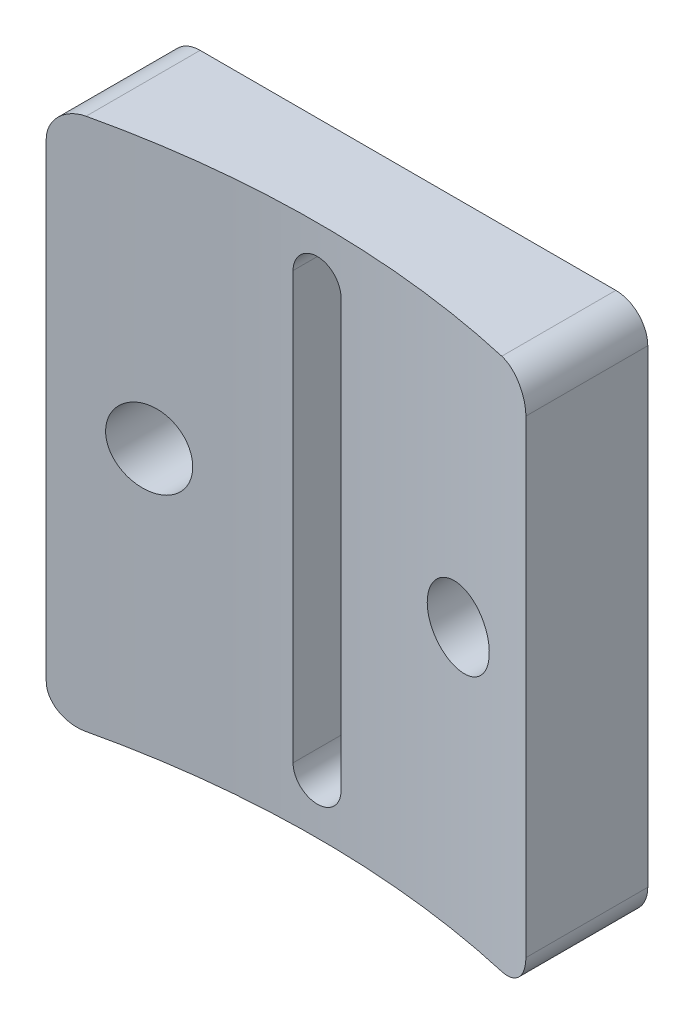
SolidWorks part; units mm, degrees
ref_plane "Front Plane" through (0, 0, 0) normal (0, 0, 1) x (1, 0, 0)
ref_plane "Top Plane" through (0, 0, 0) normal (0, 1, 0) x (1, 0, 0)
ref_plane "Right Plane" through (0, 0, 0) normal (1, 0, 0) x (0, 0, -1)
sketch "Sketch1" plane through (0, 0, 0) normal (0, 1, 0) x (1, 0, 0)
  line L0 (-22.5, 84.5577) -> (-22.5, 96)
  line L1 (-22.5, 96) -> (22.5, 96)
  line L2 (22.5, 96) -> (22.5, 84.5577)
  line L3 (0, 0) -> (0, 120.121) construction
  arc A0 (22.5, 84.5577) -> (-22.5, 84.5577) centre (0, 0) ccw
  dimension "D1" = 175
  dimension "D2" = 45
  dimension "D4" = 96
extrude "Boss-Extrude1" add sketch "Sketch1" along normal blind 50
hole_wizard "M8x1.0 Tapped Hole1" positions "Sketch3" profile "Sketch2" tap size "M8x1.0" standard "GB" end condition through all
sketch "Sketch3" plane through (0, 0, -96) normal (0, 0, -1) x (-1, 0, 0)
  line L0 (-22.5, 0) -> (22.5, 0) construction
  line L1 (22.5, 50) -> (-22.5, 50) construction
  line L2 (-22.5, 50) -> (-22.5, 0) construction
  line L3 (22.5, 50) -> (22.5, 0) construction
  point P0 (-14.5, 25)
  point P2 (14.5, 25)
  point P5 (0, 0)
  point P8 (0, 50)
  point P11 (-22.5, 25)
  point P14 (22.5, 25)
  dimension "D1" = 14.5
  dimension "D2" = 14.5
  dimension "D3" = 0
  dimension "D4" = 0
sketch "Sketch2" plane through (14.5, 25, -96) normal (1, 0, 0) x (0, 1, 0)
  line L0 (0, 0) -> (0, 11.4423)
  line L1 (0, 11.4423) -> (3.5, 11.4423)
  line L2 (3.5, 11.4423) -> (3.5, 0)
  line L5 (3.5, 0) -> (0, 0)
  line L11 (0, -6.35) -> (0, 107.95) construction
  dimension "通孔螺纹孔钻头直径" = 7
  dimension "通孔螺纹孔钻头深度" = 11.4423
cosmetic thread "Cosmetic thread 1" parameters "D1"=8.0513, "D2"=8
cosmetic thread "Cosmetic thread 2" parameters "D1"=8.0513, "D2"=8
sketch "Sketch4" plane through (0, 0, -96) normal (0, 0, -1) x (-1, 0, 0)
  line L0 (0, 0) -> (0, 35.1081) construction
  line L2 (-22.5, 25) -> (24.5658, 25) construction
  line L3 (-22.5, 50) -> (-22.5, 0) construction
  line L5 (0, 45) -> (0, 5) construction
  line L6 (2.25, 45) -> (2.25, 5)
  line L7 (-2.25, 45) -> (-2.25, 5)
  arc A2 (2.25, 45) -> (-2.25, 45) centre (0, 45) ccw
  arc A3 (-2.25, 5) -> (2.25, 5) centre (0, 5) ccw
  point P15 (0, 25)
  dimension "D6" = 2.25
  dimension "D5" = 40
extrude "Cut-Extrude1" cut sketch "Sketch4" against normal through all
sketch "Sketch5" plane through (0, 0, -96) normal (0, 0, -1) x (-1, 0, 0)
  line L0 (0, 45) -> (0, 5) construction
  line L1 (4, 45) -> (4, 5)
  line L2 (-4, 45) -> (-4, 5)
  arc A0 (4, 45) -> (-4, 45) centre (0, 45) ccw
  arc A1 (-4, 5) -> (4, 5) centre (0, 5) ccw
  point P2 (0, 25)
  dimension "D1" = 4
extrude "Cut-Extrude2" cut sketch "Sketch5" against normal blind 4
fillet "Fillet1" radius 3 4 edges at (-22.5, 50, -90.2788) (22.5, 50, -90.2788) (-22.5, 0, -90.2788) (22.5, 0, -90.2788)
